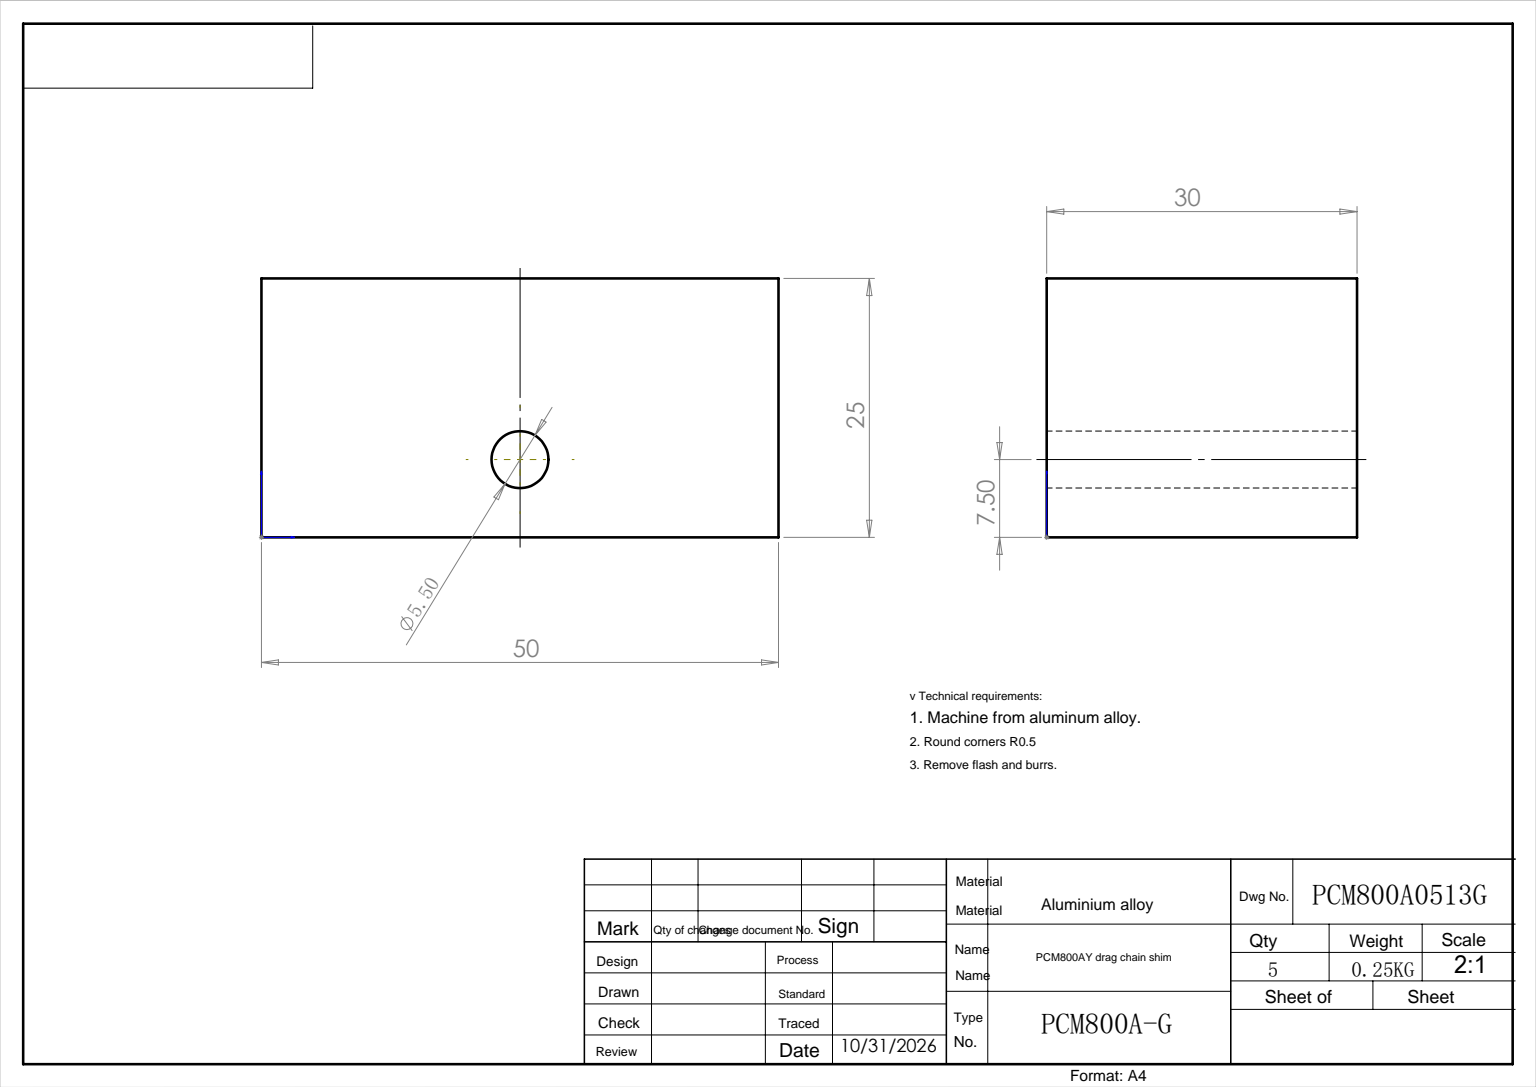
from build123d import *

# Parameters (mm, degrees)
SKETCH_1_W          = 50
SKETCH_1_H          = 25
EXTRUDE_1_DEPTH     = 30
SKETCH_2_R          = 2.75
CUT_EXTRUDE_1_DEPTH = 37


with BuildPart() as part:
    # 草图1 → 凸台-拉伸1 (new body)
    with BuildSketch(Plane.XY):
        with Locations((25, 12.5)):
            Rectangle(SKETCH_1_W, SKETCH_1_H)
    extrude(amount=EXTRUDE_1_DEPTH)

    # 草图2 → 切除-拉伸1 (cut)
    with BuildSketch(Plane.XY.offset(30)):
        with Locations((25, 7.5)):
            Circle(SKETCH_2_R)
    extrude(amount=-CUT_EXTRUDE_1_DEPTH, mode=Mode.SUBTRACT)


solid = part.part
